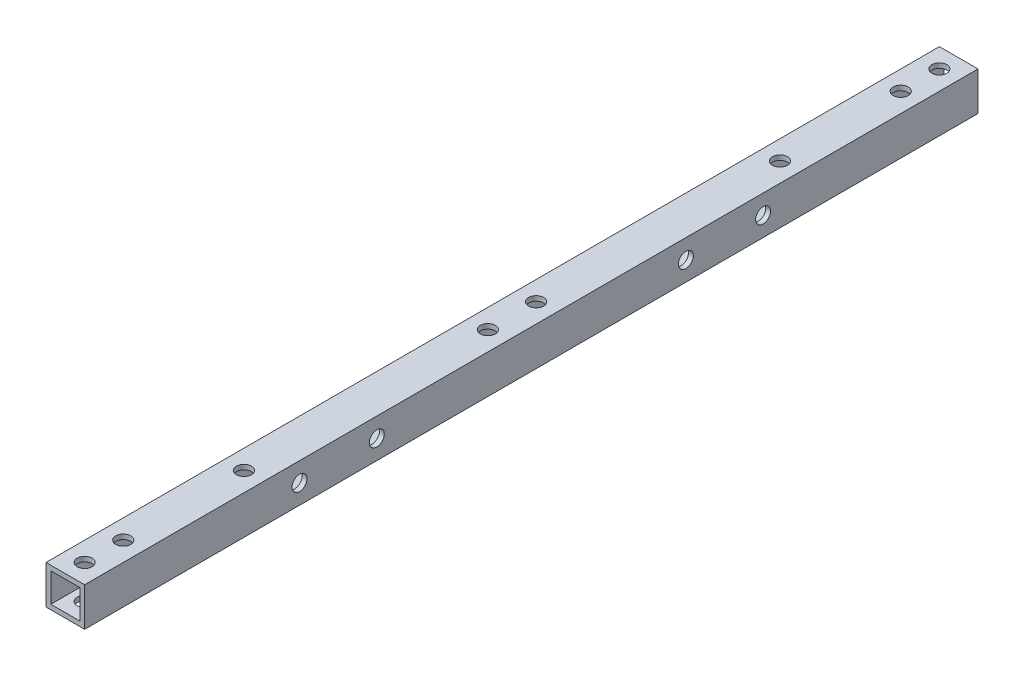
SolidWorks part; units mm, degrees
material "Thornel Mat VMA"
ref_plane "前视基准面" through (0, 0, 0) normal (0, 0, 1) x (1, 0, 0)
ref_plane "上视基准面" through (0, 0, 0) normal (0, 1, 0) x (1, 0, 0)
ref_plane "右视基准面" through (0, 0, 0) normal (1, 0, 0) x (0, 0, -1)
other "Configuration Table"
sketch "草图1" plane through (0, 0, 0) normal (0, 0, 1) x (1, 0, 0)
  line L1 (-4, 4) -> (4, 4)
  line L2 (-4, 4) -> (-4, -4)
  line L3 (-4, -4) -> (4, -4)
  line L4 (4, 4) -> (4, -4)
  line L5 (-4, 4) -> (4, -4) construction
  line L6 (-4, -4) -> (4, 4) construction
  line L7 (-3, 3) -> (3, 3)
  line L8 (-3, 3) -> (-3, -3)
  line L9 (-3, -3) -> (3, -3)
  line L10 (3, 3) -> (3, -3)
  line L11 (-3, 3) -> (3, -3) construction
  line L12 (-3, -3) -> (3, 3) construction
  point P0 (0, 0)
  point P6 (0, 0)
  dimension "D1" = 8
  dimension "D2" = 1
extrude "凸台-拉伸1" add sketch "草图1" along normal blind 185
sketch "草图2" plane through (4, 0, 0) normal (1, 0, 0) x (0, 0, -1)
  line L0 (-185, 4) -> (0, 4) construction
  line L1 (0, -4) -> (0, 4) construction
  line L2 (-92.5, 55.569) -> (-92.5, -42.8943) construction
  circle A0 centre (-44.5, 0) radius 1.55
  circle A1 centre (-60.5, 0) radius 1.55
  circle A2 centre (-124.5, 0) radius 1.55
  circle A3 centre (-140.5, 0) radius 1.55
  dimension "D1" = 3.1
  dimension "D2" = 4
  dimension "D3" = 16
  dimension "D4" = 44.5
  dimension "D5" = 92.5
extrude "切除-拉伸1" cut sketch "草图2" against normal through all
sketch "草图3" plane through (0, 4, 0) normal (0, 1, 0) x (1, 0, 0)
  line L0 (4, 0) -> (-4, 0) construction
  line L1 (4, -185) -> (-4, -185) construction
  circle A0 centre (0, -4) radius 1.55
  circle A1 centre (0, -12) radius 1.55
  circle A2 centre (0, -173) radius 1.55
  circle A3 centre (0, -181) radius 1.55
  circle A4 centre (0, -87.5) radius 1.55
  circle A5 centre (0, -97.5) radius 1.55
  circle A6 centre (0, -148) radius 1.55
  circle A7 centre (0, -37) radius 1.55
  dimension "D1" = 3.1
  dimension "D2" = 8
  dimension "D4" = 4
  dimension "D5" = 4
  dimension "D6" = 10
  dimension "D8" = 25
  dimension "D9" = 25
  dimension "D3" = 8
  dimension "D7" = 87.5
extrude "切除-拉伸2" cut sketch "草图3" against normal through all
sketch "草图4" plane through (4, 0, 0) normal (1, 0, 0) x (0, 0, -1)
  line L0 (-92.5, 17.008) -> (-92.5, -24.4266) construction
  line L1 (-185, -4) -> (-185, 4) construction
  line L2 (-185, 4) -> (0, 4) construction
  circle A0 centre (-102.5, 0) radius 1.55
  circle A1 centre (-82.5, 0) radius 1.55
  dimension "D2" = 3.1
  dimension "D3" = 4
  dimension "D4" = 10
  dimension "D1" = 92.5
extrude "切除-拉伸3" [suppressed] cut sketch "草图4" against normal blind 10
sketch "草图5" [suppressed] plane through (0, 4, 0) normal (0, 1, 0) x (1, 0, 0)
  circle A0 centre (0, -65.5) radius 1.55
  circle A1 centre (0, -97.5) radius 1.55 construction
  circle A2 centre (0, -87.5) radius 1.55 construction
  dimension "D1" = 22
extrude "切除-拉伸4" [suppressed] cut sketch "草图5" against normal blind 10
